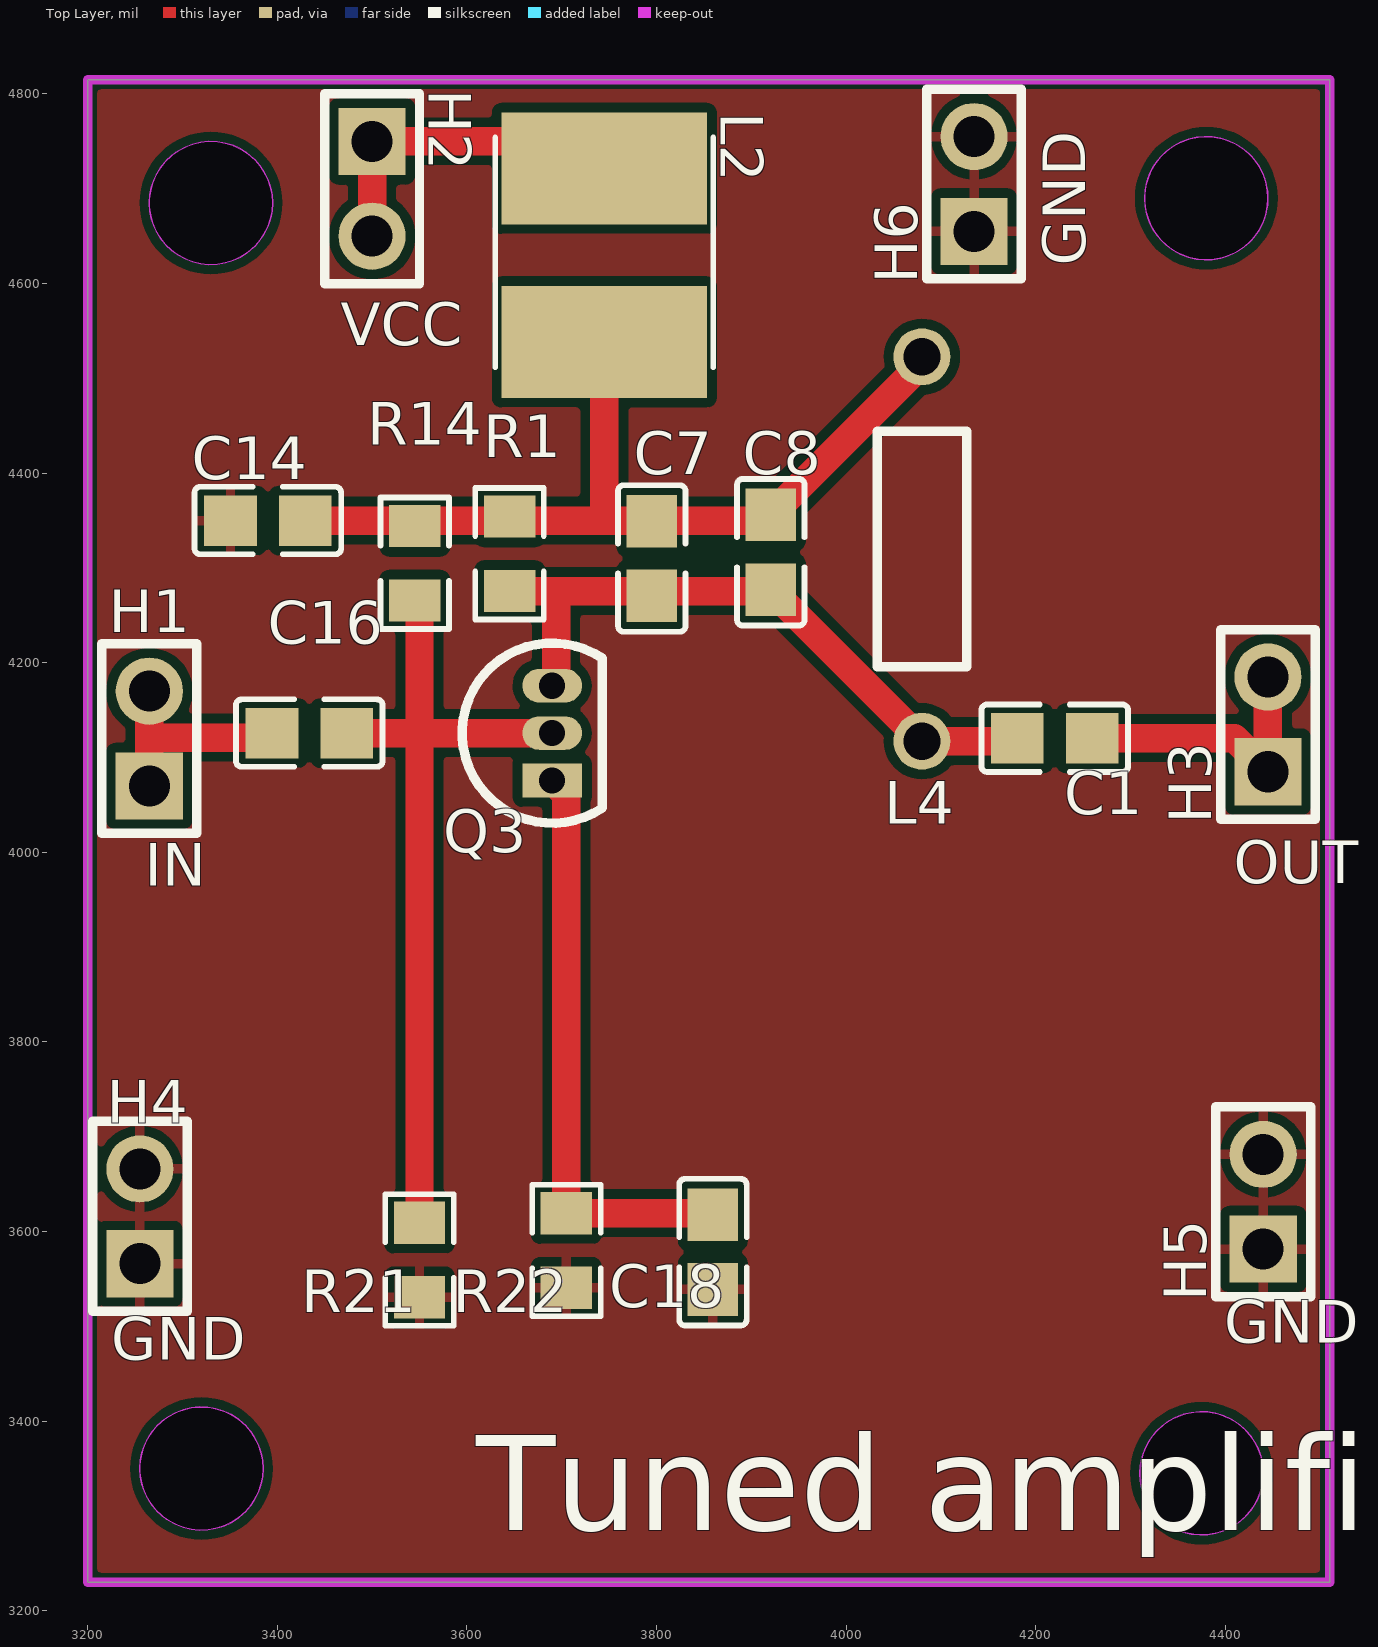
[diagram p0: Top Layer view]
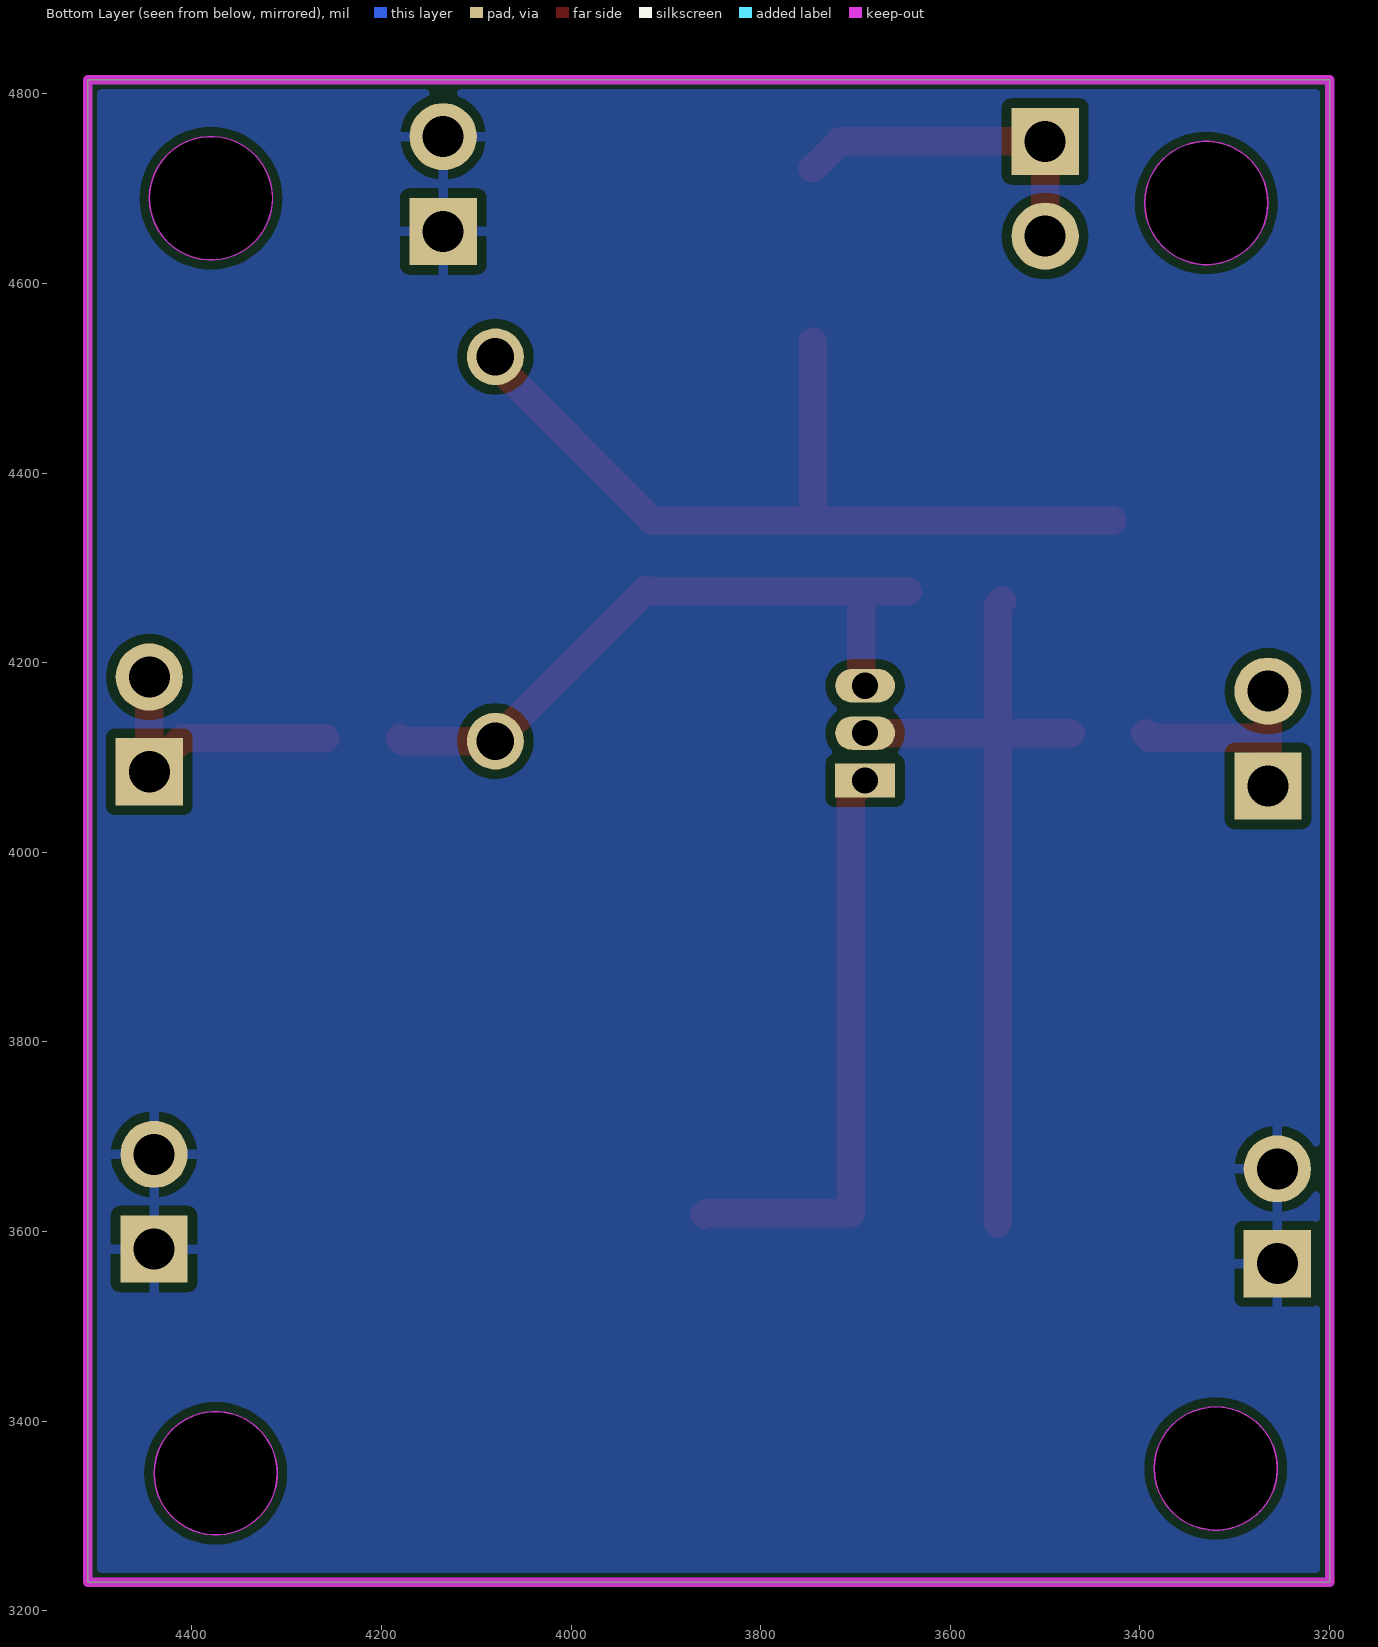
[diagram p1: Bottom Layer view, seen from below]
# Altium PCB MISC51307.pcbdoc
Units mil, origin at the board's own origin, x right, y up, seen from the top; angles counter-clockwise.
Board outline 1310 x 1585 mil, 2 copper layers (Top Layer, Bottom Layer), stack 62.206 mil thick; 19 components, 8 nets, 39 pads, 0 vias.

## Layer stack, top to bottom
Top Solder Mask Layer: solder mask 0.394, Dk 3.3
Top Layer: signal copper 1.379
Dielectric1: surface 59.449, FR4, Dk 4.5
Bottom Layer: signal copper 1.378
Bottom Solder Mask Layer: solder mask 0.394, Dk 3.3

## Board outline
3200,4815 3200,3230 4510,3230 4510,4815
cut-out: 3385,3350 cw(c3320,3350) 3255,3350 cw(c3320,3350)
cut-out: 4440,3345 cw(c4375,3345) 4310,3345 cw(c4375,3345)
cut-out: 4445,4690 cw(c4380,4690) 4315,4690 cw(c4380,4690)
cut-out: 3395,4685 cw(c3330,4685) 3265,4685 cw(c3330,4685)

## Design rules (kind name [scope] priority, off if disabled: settings)
BoardOutlineClearance copperThickness2oz_1 [All] p2 off: genericclearance=7.99 ignorepadtopadclearanceinfootprint=FALSE except(0: Arc-SplitContinuation Track-SplitContinuation SMDPad-SplitContinuation THPad-SplitContinuation Via-SplitContinuation Fill-SplitContinuation Region-SplitContinuation Poly-SplitContinuation Text-SplitContinuation Hole-SplitContinuation; 5.98: Arc-CutoutEdge SMDPad-CutoutEdge THPad-CutoutEdge Via-CutoutEdge Fill-CutoutEdge Region-CutoutEdge Text-CutoutEdge; 6.93: Hole-OutlineEdge Hole-CutoutEdge; 10: Poly-OutlineEdge Poly-CutoutEdge; 11.81: Arc-OutlineEdge Track-OutlineEdge SMDPad-OutlineEdge THPad-OutlineEdge Via-OutlineEdge Fill-OutlineEdge Region-OutlineEdge Text-OutlineEdge Track-CutoutEdge)
BoardOutlineClearance copperThickness1oz_1 [All] p4: genericclearance=4.02 ignorepadtopadclearanceinfootprint=FALSE except(0: Arc-SplitContinuation Track-SplitContinuation SMDPad-SplitContinuation THPad-SplitContinuation Via-SplitContinuation Fill-SplitContinuation Region-SplitContinuation Poly-SplitContinuation Text-SplitContinuation Hole-SplitContinuation; 6: SMDPad-CutoutEdge THPad-CutoutEdge Via-CutoutEdge Fill-CutoutEdge Region-CutoutEdge Text-CutoutEdge; 6.93: Hole-OutlineEdge Hole-CutoutEdge; 10: Poly-OutlineEdge Poly-CutoutEdge; 11.8: Arc-OutlineEdge Track-OutlineEdge SMDPad-OutlineEdge THPad-OutlineEdge Via-OutlineEdge Fill-OutlineEdge Region-OutlineEdge Text-OutlineEdge; 11.81: Arc-CutoutEdge Track-CutoutEdge)
Clearance copperThickness2oz [All] p1 off: gap=7.99 ignorepadtopadclearanceinfootprint=FALSE except(5.98: SMDPad-Track SMDPad-SMDPad THPad-Track SMDPad-THPad THPad-THPad Track-Via SMDPad-Via THPad-Via Via-Via Fill-Track Region-Track Fill-SMDPad Region-SMDPad Fill-THPad Region-THPad Fill-Via Region-Via Fill-Fill Fill-Region Region-Region Arc-Track Arc-SMDPad Arc-THPad Arc-Via Fill-Arc Region-Arc Arc-Arc Text-Track SMDPad-Text Text-THPad Text-Via Fill-Text Region-Text Arc-Text Text-Text; 6.93: Hole-Track Hole-SMDPad Hole-THPad Hole-Via Fill-Hole Region-Hole Hole-Arc Hole-Text; 10: Poly-Track Poly-SMDPad Poly-THPad Poly-Via Poly-Fill Poly-Region Poly-Poly Poly-Arc Poly-Text Poly-Hole)
Clearance copperThickness1oz [All] p3: gap=4.02 ignorepadtopadclearanceinfootprint=FALSE except(5.98: SMDPad-Track SMDPad-SMDPad THPad-Track SMDPad-THPad THPad-THPad Track-Via SMDPad-Via THPad-Via Via-Via Fill-Track Region-Track Fill-SMDPad Region-SMDPad Fill-THPad Region-THPad Fill-Via Region-Via Fill-Fill Fill-Region Region-Region; 6: Arc-Track Arc-SMDPad Arc-THPad Arc-Via Fill-Arc Region-Arc Arc-Arc Text-Track SMDPad-Text Text-THPad Text-Via Fill-Text Region-Text Arc-Text Text-Text; 6.93: Hole-Track Hole-SMDPad Hole-THPad Hole-Via Fill-Hole Region-Hole Hole-Arc Hole-Text; 10: Poly-Track Poly-SMDPad Poly-THPad Poly-Via Poly-Fill Poly-Region Poly-Poly Poly-Arc Poly-Text Poly-Hole)
Creepage creepage [All] p1: checkdistance=0 ignoreinternallayers=TRUE applytopolygonpour=TRUE
DiffPairsRouting differentialPair [All] p1: maxlimit=6 minlimit=6 mostfreqgap=6 toplayer_minwidth=5 toplayer_prefwidth=10 toplayer_maxwidth=100 toplayer_mingap=6 toplayer_prefgap=6 toplayer_maxgap=6 bottomlayer_minwidth=5 bottomlayer_prefwidth=10 bottomlayer_maxwidth=100 bottomlayer_mingap=6 bottomlayer_prefgap=6 bottomlayer_maxgap=6 maxuncoupledlength=10
HoleToHoleClearance otherClearance [All] p1: gap=11.81 allowstackedmicrovias=TRUE
Length netLength [All] p1: minlimit=0 maxlimit=0
MatchedLengths netLengthTolerance [All] p1: tolerance=1000
PasteMaskExpansion pasteMaskExpansion [All] p1: expansion=0
PlaneConnect innerPlane [All] p1: planeconnectstyle=Relief reliefexpansion=20 reliefentries=4 reliefconductorwidth=10 reliefairgap=10
PolygonConnect copperRegion [(InNet('GND'))] p1: connectstyle=Relief reliefconductorwidth=10 reliefentries=4 polygonreliefangle="90 Angle" airgapwidth=10 via.connectstyle=Relief via.reliefconductorwidth=10 via.reliefentries=4 via.polygonreliefangle="90 Angle" via.airgapwidth=10
RoutingVias viaSize [All] p1: holewidth=12.01 width=24.02 viastyle="Through Hole" minholewidth=11.81 minwidth=19.68 maxholewidth=248.03 maxwidth=393.7
SolderMaskExpansion solderMaskExpansion [IsVia] p1: expansion=-1000 istentingtop=TRUE
SolderMaskExpansion solderMaskExpansion [All] p2: expansion=2 istentingtop=FALSE
Width copperThickness2oz_2 [All] p1 off: maxlimit=100 minlimit=8 preferedwidth=10
Width copperThickness1oz_2 [All] p2: maxlimit=100 minlimit=5 preferedwidth=10

## Components (designator, comment, footprint, x,y, rotation, side; value= is the part's Value field where it differs from the comment)
C1 "100nF" C0805 4220.11,4120.37 r0 top
C7 "20pF" C0805 3795,4310 r90 top
C8 "20pF" C0805 3920.58,4316.58 r90 top
C14 "100nF" C0805 3390,4350 r0 top
C16 "100nF" C0805 3433.73,4125.79 r180 top
C18 "100nF" C0805 3859.48,3578.26 r270 top
H1 "" HDR-TH_2P-P2.54-V-M-1 3265,4120 r90 top
H2 "" HDR-TH_2P-P2.54-V-M-1 3500,4700 r270 top
H3 "" HDR-TH_2P-P2.54-V-M-1 4445,4135 r90 top
H4 "" HDR-TH_2P-P2.54-V-M-1 3255.1,3616.1 r90 top
H5 "" HDR-TH_2P-P2.54-V-M-1 4440,3631.42 r90 top
H6 "" HDR-TH_2P-P2.54-V-M-1 4135,4705 r90 top
L2 "100uH" IND-SMD_L5.8-W5.2 3745,4630 r270 top
L4 "10kΩ" Res_1/4W 4080,4320 r90 top
Q3 "" S8050_TO_92 3689.94,4125.79 r90 top
R1 "2k" R0805 3645,4315 r90 top
R14 "15k" R0805 3545,4305 r90 top
R21 "6.2k" R0805 3550,3570 r90 top
R22 "1k" R0805 3705,3580 r90 top

## Footprints (in the part's own frame and the unit in brackets; to place one, negate y for a bottom-side part, rotate by r counter-clockwise, add the part's x,y. Pads: shape width x height; smd on the part's side, far side on the other; paste and mask are expansions set on the pad)
C0805 [mm]
  rect 1.41x1.35 smd paste-100 mask+0.051: 1(-1,0) 2(1,0)
  silkscreen extent -1.96,-0.9 1.96,0.9
HDR-TH_2P-P2.54-V-M-1 [mm]
  rect 1.8x1.8 hole 1.1: 1(-1.27,0)
  round 1.8 hole 1.1: 2(1.27,0)
  silkscreen extent -2.54,-1.27 2.54,1.27
IND-SMD_L5.8-W5.2 [mm]
  rect 3x5.5 smd paste-100 mask+0.05: 1(2.325,0) 2(-2.325,0)
  silkscreen extent -3.15,-2.92 3,2.92
R0805 [mm]
  rect 1.133x1.377 smd paste-100 mask+0.051: 1(-1,0) 2(1,0)
  silkscreen extent -1.76,-0.92 1.76,0.92
Res_1/4W [mil]
  round 60 hole 39.37 paste+0 mask+2: 1(-202.76,0) 2(202.76,0)
  silkscreen extent -124,-47 124,47
S8050_TO_92 [mil]
  rect 35.4x63 hole 27.6 paste+0 mask+2: 1(-50,0)
  oval 35.4x63 hole 27.6 paste+0 mask+2: 2(0,0) 3(50,0)
  silkscreen extent -95,-53 95,95

## Nets (pads, with @x,y where several pads share a name; then routed paths per layer and width w, separated by ;. In a path a pad name is that pad's centre, name@x,y a point inside that pad or via, vN(x,y) a via of type N, cw(c..) or ccw(c..) an arc to the next point about the centre after c; other vN are vias at no path point)
$1N1: C16.2 H1.1 H1.2 | length 231.4
  Top Layer w30: H1.1 3265,4120.93 ; H1.2 3265,4120.93 ; C16.2 3389.5,4120.93 3265,4120.93
$1N2: C16.1 Q3.2 R14.1 R21.2 | length 875.2
  Top Layer w30: C16.1 3550,4125.79 ; R14.1 3550,4260.63 3550,4125.79 ; R21.2 3550,4125.79 ; Q3.2 3550,4125.79
$1N4: C18.1 Q3.1 R22.2 | length 617.9
  Top Layer w30: Q3.1 3705,4060.73 R22.2 3857.74,3619.37 C18.1
$1N5: C1.1 C7.1 C8.1 L4.1 Q3.3 R1.1 | length 705.8
  Top Layer w30: R1.1 3694.03,4275.63 ; Q3.3 3694.03,4179.88 3694.03,4275.63 ; C1.1 4177.61,4117.24 L4.1 4080,4117.78 C8.1 3919,4275.63 3694.03,4275.63
$1N6: C7.2 C8.2 C14.2 L2.1 L4.2 R1.2 R14.2 | length 915.4
  Top Layer w30: C14.2 3745.94,4350 ; L2.1 3745,4350.94 3745.94,4350 ; L4.2 4080,4515.37 C8.2 3914.63,4350 3745.94,4350
$1N8: H2.1 H2.2 L2.2 | length 356.8
  Top Layer w30: H2.2 H2.1 3716.55,4750 L2.2
$1N9: C1.2 H3.1 H3.2 | length 300.2
  Top Layer w30: C1.2 4409.63,4120.37 H3.1 H3.2
GND: C14.1 C18.2 H4.1 H4.2 H5.1 H5.2 H6.1 H6.2 R21.1 R22.1

## Polygon pours and split planes (outlines as drawn)
GND on Top Layer (solid, remove dead copper, pour order 0): 3000,4955 3000,3000 4700,3000 4700,4955
GND on Bottom Layer (solid, remove dead copper, pour order 2): 3105,4910 3105,3175 4660,3175 4660,4910

## Keep-outs
Board Outline Layer:
  region: 3385,3350 cw(c3320,3350) 3255,3350 cw(c3320,3350)
  circle w0.1: c3320,3350 r65
  region: 3385,3350 3384.62,3342.97 3383.48,3336.03 3381.6,3329.25 3378.99,3322.71 3375.7,3316.49 3371.75,3310.66 3367.19,3305.3 3362.08,3300.46 3356.48,3296.2 3350.45,3292.57 3344.06,3289.62 3337.39,3287.37 3330.52,3285.86 3323.52,3285.1 3316.48,3285.1 3309.48,3285.86 3302.61,3287.37 3295.94,3289.62 3289.55,3292.57 3283.52,3296.2 3277.92,3300.46 3272.81,3305.3 3268.25,3310.66 3264.3,3316.49 3261.01,3322.71 3258.4,3329.25 3256.52,3336.03 3255.38,3342.97 3255,3350 3255.38,3357.03 3256.52,3363.97 3258.4,3370.75 3261.01,3377.29 3264.3,3383.51 3268.25,3389.34 3272.81,3394.7 3277.92,3399.54 3283.52,3403.8 3289.55,3407.43 3295.94,3410.38 3302.61,3412.63 3309.48,3414.14 3316.48,3414.9 3323.52,3414.9 3330.52,3414.14 3337.39,3412.63 3344.06,3410.38 3350.45,3407.43 3356.48,3403.8 3362.08,3399.54 3367.19,3394.7 3371.75,3389.34 3375.7,3383.51 3378.99,3377.29 3381.6,3370.75 3383.48,3363.97 3384.62,3357.03
  region: 4440,3345 cw(c4375,3345) 4310,3345 cw(c4375,3345)
  circle w0.1: c4375,3345 r65
  region: 4440,3345 4439.62,3337.97 4438.48,3331.03 4436.6,3324.25 4433.99,3317.71 4430.7,3311.49 4426.75,3305.66 4422.19,3300.3 4417.08,3295.46 4411.48,3291.2 4405.45,3287.57 4399.06,3284.62 4392.39,3282.37 4385.52,3280.86 4378.52,3280.1 4371.48,3280.1 4364.48,3280.86 4357.61,3282.37 4350.94,3284.62 4344.55,3287.57 4338.52,3291.2 4332.92,3295.46 4327.81,3300.3 4323.25,3305.66 4319.3,3311.49 4316.01,3317.71 4313.4,3324.25 4311.52,3331.03 4310.38,3337.97 4310,3345 4310.38,3352.03 4311.52,3358.97 4313.4,3365.75 4316.01,3372.29 4319.3,3378.51 4323.25,3384.34 4327.81,3389.7 4332.92,3394.54 4338.52,3398.8 4344.55,3402.43 4350.94,3405.38 4357.61,3407.63 4364.48,3409.14 4371.48,3409.9 4378.52,3409.9 4385.52,3409.14 4392.39,3407.63 4399.06,3405.38 4405.45,3402.43 4411.48,3398.8 4417.08,3394.54 4422.19,3389.7 4426.75,3384.34 4430.7,3378.51 4433.99,3372.29 4436.6,3365.75 4438.48,3358.97 4439.62,3352.03
  region: 4445,4690 cw(c4380,4690) 4315,4690 cw(c4380,4690)
  circle w0.1: c4380,4690 r65
  region: 4445,4690 4444.62,4682.97 4443.48,4676.03 4441.6,4669.25 4438.99,4662.71 4435.7,4656.49 4431.75,4650.66 4427.19,4645.3 4422.08,4640.46 4416.48,4636.2 4410.45,4632.57 4404.06,4629.62 4397.39,4627.37 4390.52,4625.86 4383.52,4625.1 4376.48,4625.1 4369.48,4625.86 4362.61,4627.37 4355.94,4629.62 4349.55,4632.57 4343.52,4636.2 4337.92,4640.46 4332.81,4645.3 4328.25,4650.66 4324.3,4656.49 4321.01,4662.71 4318.4,4669.25 4316.52,4676.03 4315.38,4682.97 4315,4690 4315.38,4697.03 4316.52,4703.97 4318.4,4710.75 4321.01,4717.29 4324.3,4723.51 4328.25,4729.34 4332.81,4734.7 4337.92,4739.54 4343.52,4743.8 4349.55,4747.43 4355.94,4750.38 4362.61,4752.63 4369.48,4754.14 4376.48,4754.9 4383.52,4754.9 4390.52,4754.14 4397.39,4752.63 4404.06,4750.38 4410.45,4747.43 4416.48,4743.8 4422.08,4739.54 4427.19,4734.7 4431.75,4729.34 4435.7,4723.51 4438.99,4717.29 4441.6,4710.75 4443.48,4703.97 4444.62,4697.03
  region: 3395,4685 cw(c3330,4685) 3265,4685 cw(c3330,4685)
  circle w0.1: c3330,4685 r65
  region: 3395,4685 3394.62,4677.97 3393.48,4671.03 3391.6,4664.25 3388.99,4657.71 3385.7,4651.49 3381.75,4645.66 3377.19,4640.3 3372.08,4635.46 3366.48,4631.2 3360.45,4627.57 3354.06,4624.62 3347.39,4622.37 3340.52,4620.86 3333.52,4620.1 3326.48,4620.1 3319.48,4620.86 3312.61,4622.37 3305.94,4624.62 3299.55,4627.57 3293.52,4631.2 3287.92,4635.46 3282.81,4640.3 3278.25,4645.66 3274.3,4651.49 3271.01,4657.71 3268.4,4664.25 3266.52,4671.03 3265.38,4677.97 3265,4685 3265.38,4692.03 3266.52,4698.97 3268.4,4705.75 3271.01,4712.29 3274.3,4718.51 3278.25,4724.34 3282.81,4729.7 3287.92,4734.54 3293.52,4738.8 3299.55,4742.43 3305.94,4745.38 3312.61,4747.63 3319.48,4749.14 3326.48,4749.9 3333.52,4749.9 3340.52,4749.14 3347.39,4747.63 3354.06,4745.38 3360.45,4742.43 3366.48,4738.8 3372.08,4734.54 3377.19,4729.7 3381.75,4724.34 3385.7,4718.51 3388.99,4712.29 3391.6,4705.75 3393.48,4698.97 3394.62,4692.03
  lines w10: 3200,3230 3200,4815 4510,4815 4510,3230 3200,3230

## Silkscreen, mask and mechanical layers (free items; w line width, h text height)
Top Silkscreen Layer:
  text "GND" at 4252.5,4618.95 h45 r90
  text "VCC" at 3466.75,4534.77 h45
  text "OUT" at 4408.95,3967.5 h45
  text "IN" at 3260,3965 h45
  text "GND" at 4398.95,3482.82 h45
  text "GND" at 3225,3465 h45
  text "Tuned amplifier" at 3610,3285 h100
Mechanical Layer:
  circle w0.1: c3320,3350 r65
  circle w0.1: c4375,3345 r65
  circle w0.1: c4380,4690 r65
  circle w0.1: c3330,4685 r65